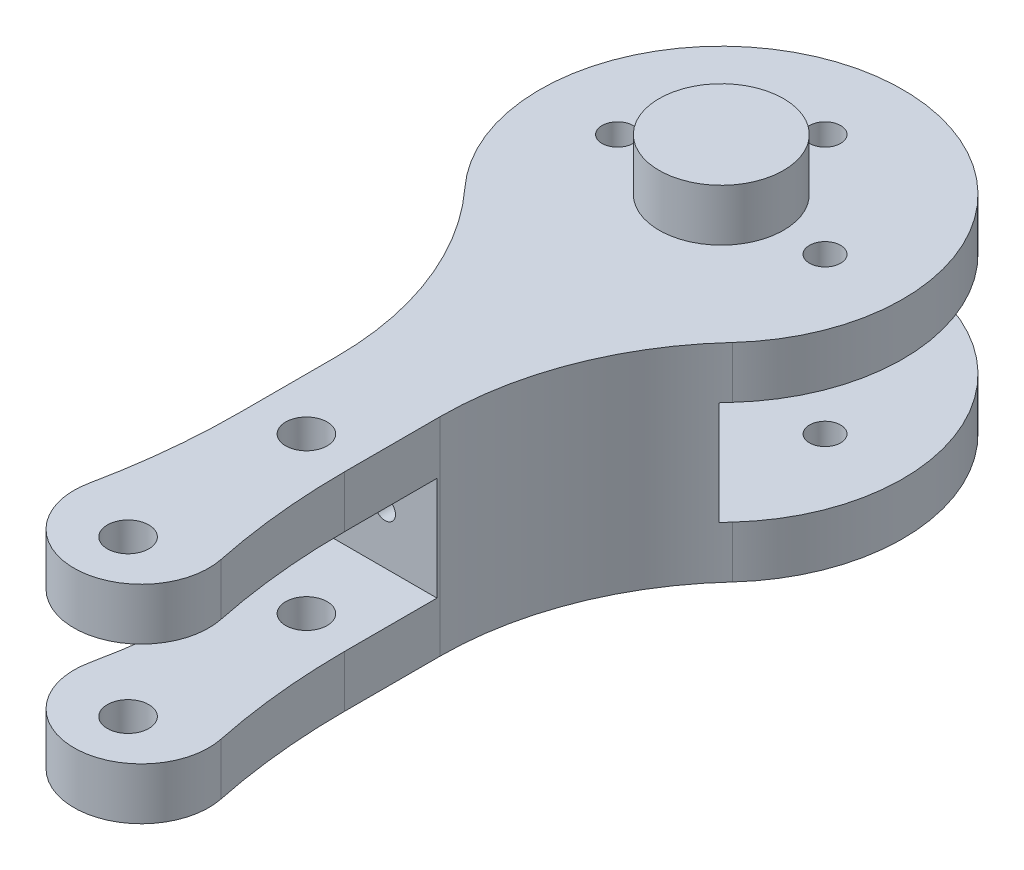
SolidWorks part; units mm, degrees
ref_plane "Front Plane" through (0, 0, 0) normal (0, 0, 1) x (1, 0, 0)
ref_plane "Top Plane" through (0, 0, 0) normal (0, 1, 0) x (1, 0, 0)
ref_plane "Right Plane" through (0, 0, 0) normal (1, 0, 0) x (0, 0, -1)
other "Configuration Table"
sketch "Sketch1" plane through (0, 0, 0) normal (0, 1, 0) x (1, 0, 0)
  line L0 (0, 0) -> (0, -61.3733) construction
  line L1 (-5, -32.1131) -> (-5, -41.3465)
  line L2 (5, -32.1131) -> (5, -41.3465)
  arc A1 (-12.8947, -11.8311) -> (-5, -32.1131) centre (-35, -32.1131) cw
  arc A2 (12.8947, -11.8311) -> (5, -32.1131) centre (35, -32.1131) ccw
  arc A3 (-6.3636, -54.5909) -> (6.3636, -54.5909) centre (0, -55.9153) ccw
  arc A4 (12.8947, -11.8311) -> (-12.8947, -11.8311) centre (0, 0) ccw
  arc A5 (-5, -41.3465) -> (-6.3636, -54.5909) centre (-70, -41.3465) cw
  arc A6 (5, -41.3465) -> (6.3636, -54.5909) centre (70, -41.3465) ccw
  dimension "D1" = 65
  dimension "D3" = 30
  dimension "D4" = 13
  dimension "D2" = 5
extrude "Boss-Extrude1" add sketch "Sketch1" along normal blind 20
sketch "Sketch2" plane through (0, 20, 0) normal (0, 1, 0) x (1, 0, 0)
  circle A0 centre (0, -40) radius 2
  circle A1 centre (0, -57.194) radius 2
  dimension "D2" = 4
  dimension "D3" = 4
  dimension "D1" = 40
extrude "Cut-Extrude1" cut sketch "Sketch2" against normal through all both and the other way through all
sketch "Sketch3" plane through (0, 20, 0) normal (0, 1, 0) x (1, 0, 0)
  circle A0 centre (0, 0) radius 2
  dimension "D1" = 4
extrude "Cut-Extrude2" cut sketch "Sketch3" against normal through all
sketch "Sketch4" plane through (0, 20, 0) normal (0, 1, 0) x (1, 0, 0)
  line L0 (0, 0) -> (-50000, 0) construction
  line L1 (0, 0) -> (0, -50000) construction
  circle A0 centre (-10, 0) radius 1.5
  circle A1 centre (10, 0) radius 1.5
  circle A2 centre (0, 10) radius 1.5
  dimension "D1" = 3
  dimension "D2" = 3
  dimension "D3" = 3
  dimension "D4" = 10
  dimension "D5" = 10
  dimension "D6" = 10
extrude "Cut-Extrude3" cut sketch "Sketch4" against normal through all
sketch "Sketch5" plane through (0, 0, 0) normal (1, 0, 0) x (0, 0, -1)
  line L0 (-62.4153, 15) -> (-32.4153, 15)
  line L1 (-62.4153, 20) -> (-62.4153, 0) construction
  line L2 (-32.4153, 15) -> (-32.4153, 5)
  line L3 (-32.4153, 5) -> (-62.4153, 5)
  line L4 (-62.4153, 5) -> (-62.4153, 15)
  line L5 (-41.3465, 20) -> (-54.5909, 20) construction
  line L6 (-54.5909, 0) -> (-41.3465, 0) construction
  line L7 (-62.4153, 20) -> (17.5, 20) construction
  line L8 (-22.4577, 20) -> (-22.4577, 74.6443) construction
  line L9 (17.5, 5) -> (17.5, 15)
  line L10 (-12.5, 5) -> (17.5, 5)
  line L11 (-12.5, 15) -> (-12.5, 5)
  line L12 (17.5, 15) -> (-12.5, 15)
  dimension "D1" = 5
  dimension "D2" = 5
  dimension "D3" = 30
extrude "Cut-Extrude4" cut sketch "Sketch5" against normal through all both and the other way through all
sketch "Sketch6" plane through (0, 0, 0) normal (0, -1, 0) x (1, 0, 0)
  circle A0 centre (0, 0) radius 6
  dimension "D1" = 12
extrude "Boss-Extrude2" add sketch "Sketch6" against normal blind 5 from surface at -20 starting at face at (-10, 20, 1.5)
sketch "Sketch7" plane through (0, 5, 0) normal (0, 1, 0) x (1, 0, 0)
  circle A0 centre (0, 0) radius 2
extrude "Boss-Extrude4" add sketch "Sketch7" along normal up to surface (10 mm away) separate body up to face at (0, 15, -8.5)
sketch "Sketch8" plane through (0, 0, 12.5) normal (0, 0, -1) x (-1, 0, 0)
  circle A0 centre (0, 9.9758) radius 1
  dimension "D1" = 2
extrude "Cut-Extrude5" cut sketch "Sketch8" against normal blind 30
